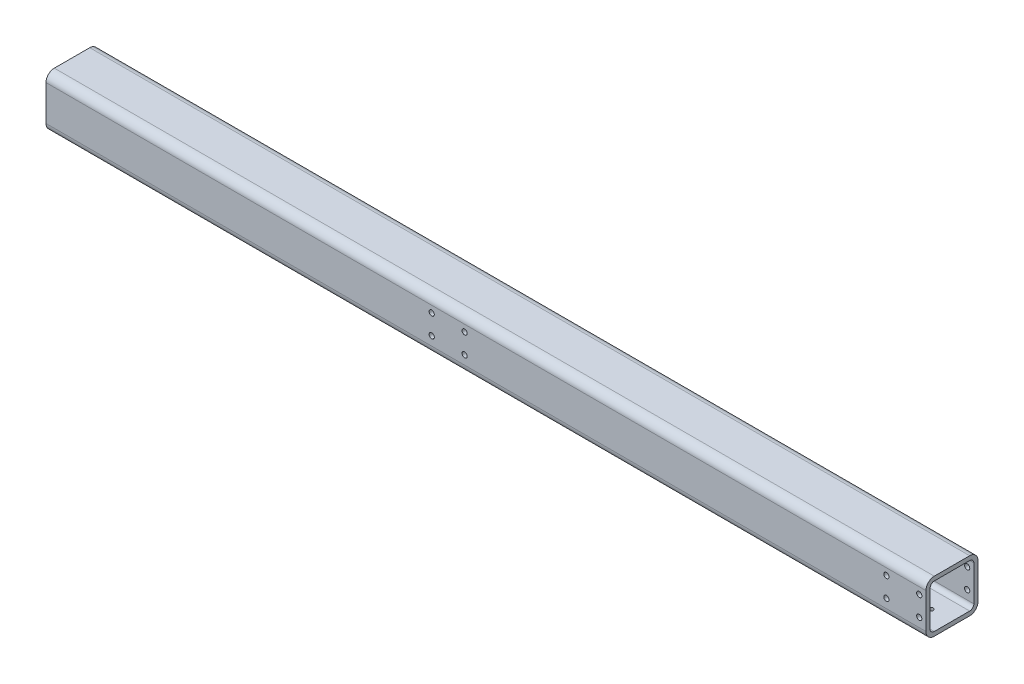
from build123d import *

# Parameters (mm, degrees)
GB_6728_1986_050_X_50_X_4_1_DEPTH = 845
HOLE_WIZARD_M6_1_D                = 5
HOLE_WIZARD_M5_1_D                = 4.2
HOLE_WIZARD_M5_1_DEPTH            = 4


with BuildPart() as part:
    # Sketch1 → Gb／6728-1986方形空心型钢 050 X 50 X 4(1) (new body)
    with BuildSketch(Plane.ZY):
        with BuildLine():
            Line((-17, -25), (17, -25))
            ThreePointArc((17, -25), (22.656854249, -22.656854249), (25, -17))
            Line((25, -17), (25, 17))
            ThreePointArc((25, 17), (22.656854249, 22.656854249), (17, 25))
            Line((17, 25), (-17, 25))
            ThreePointArc((-17, 25), (-22.656854249, 22.656854249), (-25, 17))
            Line((-25, 17), (-25, -17))
            ThreePointArc((-25, -17), (-22.656854249, -22.656854249), (-17, -25))
        make_face()
        with BuildLine():
            Line((-17, -21), (17, -21))
            ThreePointArc((17, -21), (19.828427125, -19.828427125), (21, -17))
            Line((21, -17), (21, 17))
            ThreePointArc((21, 17), (19.828427125, 19.828427125), (17, 21))
            Line((17, 21), (-17, 21))
            ThreePointArc((-17, 21), (-19.828427125, 19.828427125), (-21, 17))
            Line((-21, 17), (-21, -17))
            ThreePointArc((-21, -17), (-19.828427125, -19.828427125), (-17, -21))
        make_face(mode=Mode.SUBTRACT)
    extrude(amount=GB_6728_1986_050_X_50_X_4_1_DEPTH)

    # M6 螺纹孔1 (through all)
    with Locations(Plane(origin=(0, 0, -25), x_dir=(-1, 0, 0), z_dir=(0, 0, -1))):
        with Locations((6.4, 10.6), (6.4, -8.4), (38, 10.6), (38, -8.4), (443, 10.6), (443, -8.4), (474.6, 10.6), (474.6, -8.4)):
            Hole(HOLE_WIZARD_M6_1_D / 2)

    # M5 螺纹孔1
    with Locations(Plane(origin=(0, -25, 0), x_dir=(-1, 0, 0), z_dir=(0, -1, 0))):
        with Locations((20, 0), (190, 0), (360, 0), (530, 0)):
            Hole(HOLE_WIZARD_M5_1_D / 2, depth=HOLE_WIZARD_M5_1_DEPTH)


solid = part.part
